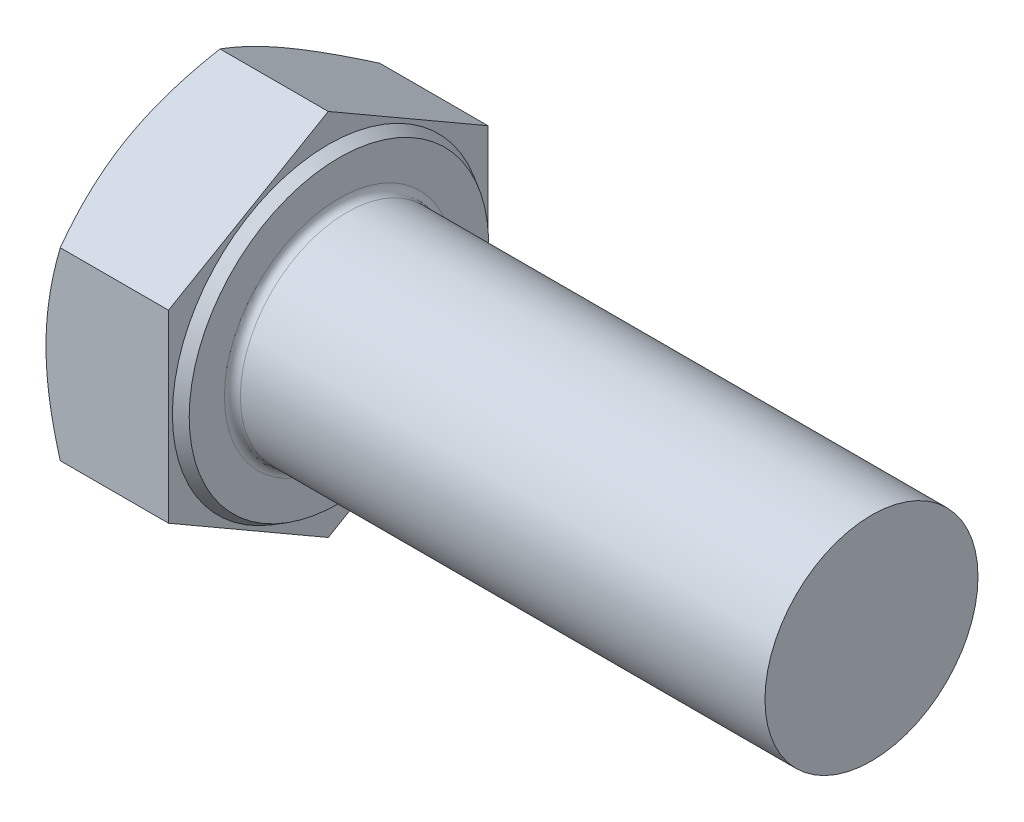
from build123d import *

# Parameters (mm, degrees)
EXTRUDE_387_DEPTH = 10
FILLET_1280_R     = 0.6


with BuildPart() as part:
    # 草图1 → Extrude 387 (new body)
    with BuildSketch(Plane(origin=(0, 0, 0), x_dir=(0, 0, -1), z_dir=(1, 0, 0))):
        Polygon((12, 6.92820323), (12, -6.92820323), (0, -13.856406461), (-12, -6.92820323), (-12, 6.92820323), (0, 13.856406461), align=None)
    extrude(amount=EXTRUDE_387_DEPTH)

    # 草图2 → 凸台-旋转1 (revolve)
    with BuildSketch(Plane.XY, mode=Mode.PRIVATE) as revolve_1_sk:
        Polygon((0, 0), (50, 0), (50, 6.268), (50, 8), (12, 8), (0, 8), align=None)
    revolve(revolve_1_sk.sketch.rotate(Axis((0, 0, 0), (1, 0, 0)), 90), axis=Axis((0, 0, 0), (1, 0, 0)))

    # 草图3 → 切除-旋转1 (revolve, cut)
    with BuildSketch(Plane.XY):
        Polygon((0, 12), (3.958548116, 18.856406461), (3.958548116, 23.856406461), (-10, 23.856406461), (-10, 12), align=None)
    revolve(axis=Axis((0, 0, 0), (1, 0, 0)), mode=Mode.SUBTRACT)

    # 草图4 → 切除-旋转3 (revolve, cut)
    with BuildSketch(Plane.XY, mode=Mode.PRIVATE) as cut_revolve_3_sk:
        Polygon((10, 11.245), (9.2, 11.706880215), (9.2, 13.856406461), (10, 13.856406461), align=None)
    revolve(cut_revolve_3_sk.sketch.rotate(Axis((0, 0, 0), (1, 0, 0)), 90), axis=Axis((0, 0, 0), (1, 0, 0)), mode=Mode.SUBTRACT)

    # Fillet 1280
    fillet_1280_edges = [part.edges().sort_by_distance(p)[0] for p in [
        (10, 0, -8),
    ]]
    fillet(fillet_1280_edges, radius=FILLET_1280_R)


solid = part.part
